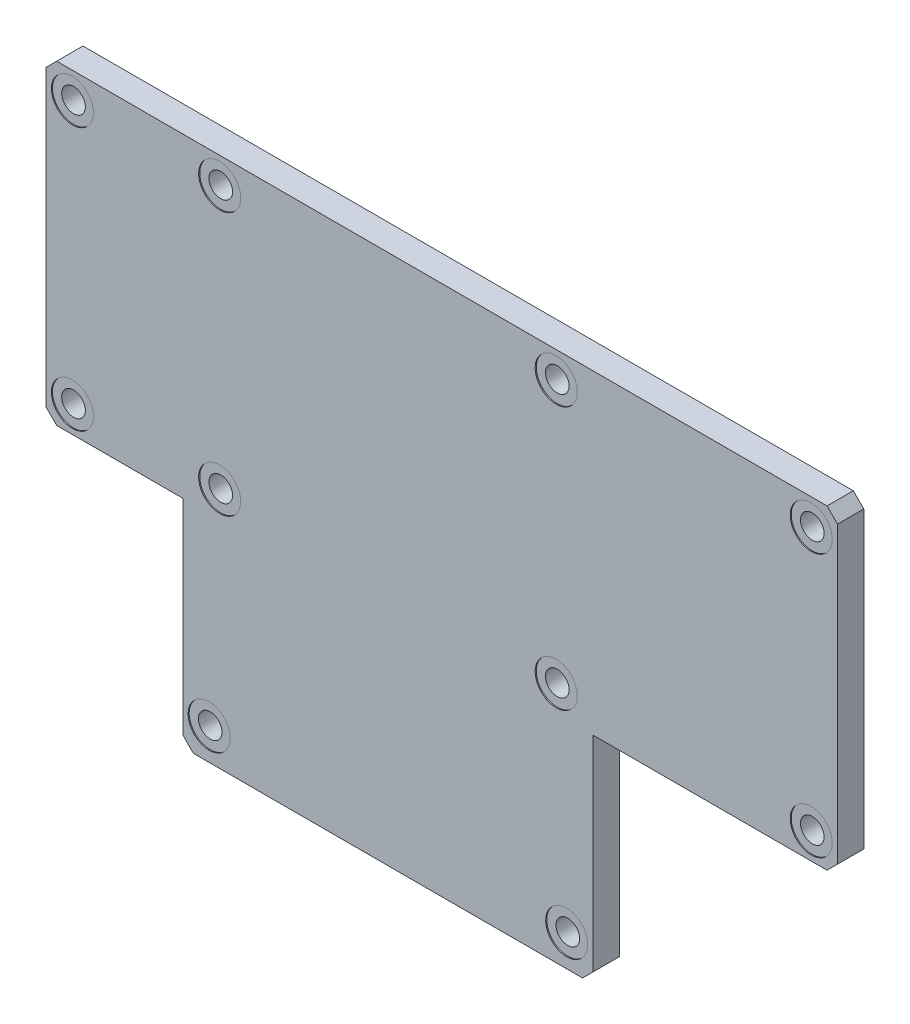
SolidWorks part; units mm, degrees
ref_plane "Front Plane" through (0, 0, 0) normal (0, 0, 1) x (1, 0, 0)
ref_plane "Top Plane" through (0, 0, 0) normal (0, 1, 0) x (1, 0, 0)
ref_plane "Right Plane" through (0, 0, 0) normal (1, 0, 0) x (0, 0, -1)
sketch "Sketch1" plane through (0, 0, 0) normal (0, 0, 1) x (1, 0, 0)
  line L0 (390, 410) -> (855, 410)
  line L2 (390, 410) -> (390, 0)
  line L3 (390, 0) -> (-390, 0)
  line L4 (-390, 410) -> (-390, 0)
  line L5 (0, 1010) -> (0, -985.8487) construction
  line L6 (0, -985.8487) -> (119.3801, -985.8487) construction
  line L7 (-650, 410) -> (-390, 410)
  line L8 (-650, 410) -> (-650, 1010)
  line L9 (-650, 1010) -> (855, 1010)
  line L10 (855, 410) -> (855, 1010)
  line L11 (855, 710) -> (-650, 710) construction
  point P0 (0, 0)
  dimension "D1" = 390
  dimension "D2" = 780
  dimension "D3" = 300
  dimension "D4" = 1010
  dimension "D5" = 1505
  dimension "D6" = 650
extrude "Boss-Extrude1" add sketch "Sketch1" along normal blind 50
hole_wizard "Hole1" positions "Sketch2" profile "Sketch3" legacy end condition through all
sketch "Sketch2" plane through (0, 0, 50) normal (0, 0, 1) x (1, 0, 0)
  line L0 (-650, 1010) -> (-650, 410) construction
  line L1 (855, 410) -> (855, 1010) construction
  line L2 (0, 1010) -> (0, -985.8487) construction
  line L3 (-650, 960) -> (855, 960) construction
  line L4 (-650, 410) -> (-650, 1010) construction
  line L5 (855, 410) -> (855, 1010) construction
  line L7 (-390, 60) -> (390, 60) construction
  line L8 (-390, 410) -> (-390, 0) construction
  line L9 (390, 410) -> (390, 0) construction
  line L11 (-650, 710) -> (855, 710) construction
  point P0 (-600, 960)
  point P4 (320, 960)
  point P6 (805, 960)
  point P8 (-340, 60)
  point P10 (340, 60)
  point P21 (-320, 960)
  point P54 (805, 460)
  point P55 (320, 460)
  point P56 (-320, 460)
  point P57 (-600, 460)
  dimension "D1" = 50
  dimension "D2" = 320
  dimension "D3" = 50
  dimension "D4" = 485
  dimension "D5" = 320
  dimension "D6" = 280
  dimension "D7" = 250
  dimension "D8" = 340
  dimension "D9" = 340
  dimension "D10" = 400
sketch "Sketch3" plane through (-600, 960, 50) normal (1, 0, 0) x (0, -1, 0)
  line L0 (0, 0) -> (0, 50)
  line L1 (0, 50) -> (22.5, 50)
  line L2 (22.5, 50) -> (22.5, 2)
  line L3 (22.5, 2) -> (40, 2)
  line L4 (40, 2) -> (40, 0)
  line L5 (40, 0) -> (0, 0)
  line L6 (0, 110) -> (0, -10) construction
  dimension "直径" = 45
  dimension "深度" = 50
  dimension "柱坑直径" = 80
  dimension "柱坑深度" = 2
chamfer "Chamfer1" distance 20 angle 45 6 edges at (-390, 0, 25) (-650, 410, 25) (390, 0, 25) (855, 410, 25) (855, 1010, 25) (-650, 1010, 25)
